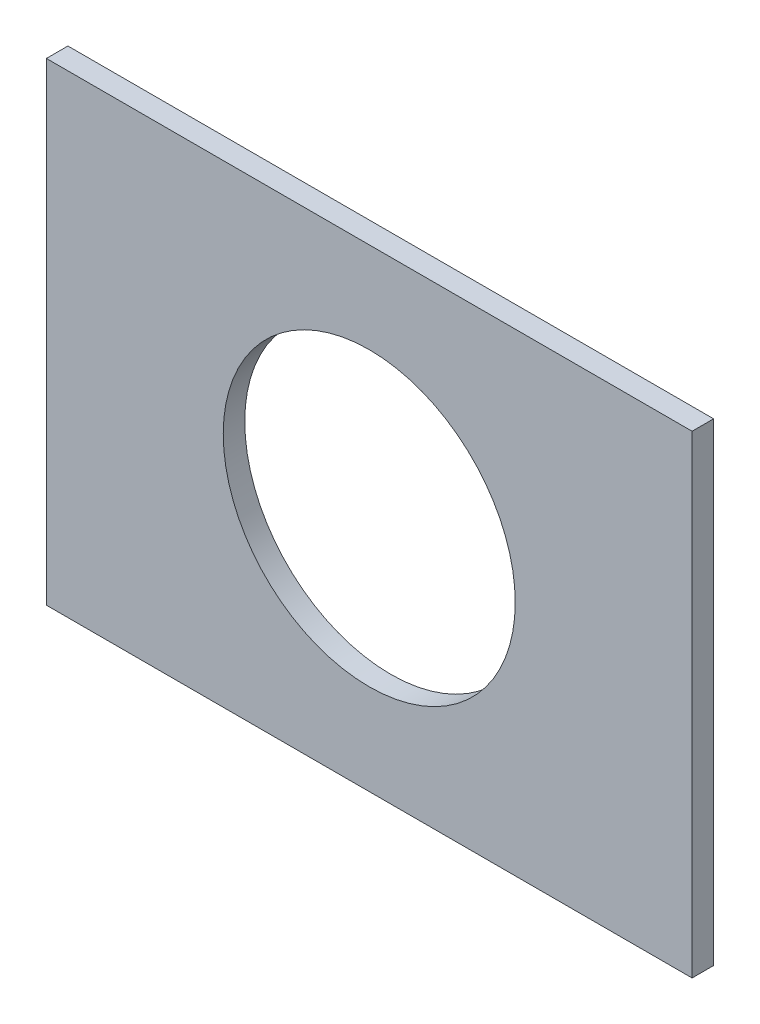
from build123d import *

# Parameters (mm, degrees)
SKETCH_1_W          = 150
SKETCH_1_H          = 110
EXTRUDE_1_DEPTH     = 2.5
SKETCH_2_R          = 33.915864145
CUT_EXTRUDE_1_DEPTH = 10


with BuildPart() as part:
    # 草图1 → 凸台-拉伸1 (new, symmetric)
    with BuildSketch(Plane.XY):
        Rectangle(SKETCH_1_W, SKETCH_1_H)
    extrude(amount=EXTRUDE_1_DEPTH, both=True)

    # 草图2 → 切除-拉伸1 (cut)
    with BuildSketch(Plane(origin=(0, 0, -2.5), x_dir=(-1, 0, 0), z_dir=(0, 0, -1))):
        Circle(SKETCH_2_R)
    extrude(amount=-CUT_EXTRUDE_1_DEPTH, mode=Mode.SUBTRACT)


solid = part.part
